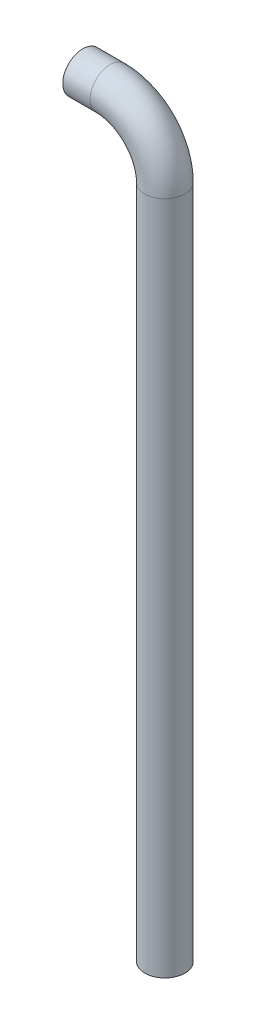
from build123d import *

# Parameters (mm, degrees)
SKETCH_2_R   = 11
SKETCH_2_R_2 = 8


with BuildPart() as part:
    # Sweep 1: sweep along a path in Sketch 1
    with BuildLine(Plane.XY) as sweep_1_path:
        Line((0, 0), (15, 0))
        ThreePointArc((15, 0), (36.213203436, -8.786796564), (45, -30))
        Line((45, -30), (45, -400))
    # Sketch 2 → Sweep 1 (sweep)
    with BuildSketch(Plane(origin=(0, 0, 0), x_dir=(0, 0, -1), z_dir=(1, 0, 0))):
        Circle(SKETCH_2_R)
        Circle(SKETCH_2_R_2, mode=Mode.SUBTRACT)
    sweep(path=sweep_1_path.line)


solid = part.part
